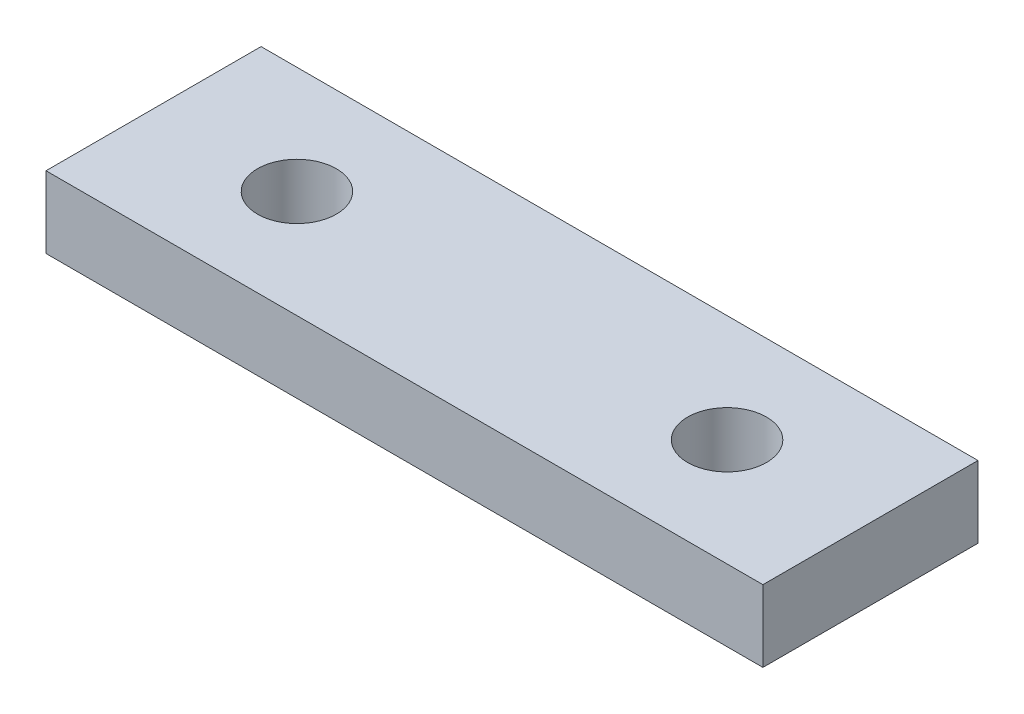
SolidWorks part; units mm, degrees
material "Q235B"
ref_plane "Front Plane" through (0, 0, 0) normal (0, 0, 1) x (1, 0, 0)
ref_plane "Top Plane" through (0, 0, 0) normal (0, 1, 0) x (1, 0, 0)
ref_plane "Right Plane" through (0, 0, 0) normal (1, 0, 0) x (0, 0, -1)
sketch "Sketch1" plane through (0, 0, 0) normal (0, 1, 0) x (1, 0, 0)
  line L1 (50, -15) -> (-50, -15)
  line L2 (50, -15) -> (50, 15)
  line L3 (50, 15) -> (-50, 15)
  line L4 (-50, -15) -> (-50, 15)
  line L5 (50, -15) -> (-50, 15) construction
  line L6 (50, 15) -> (-50, -15) construction
  point P0 (0, 0)
  dimension "D1" = 30
  dimension "D2" = 100
extrude "Boss-Extrude1" add sketch "Sketch1" along normal blind 10
hole_wizard "Ø11.0 (11) Diameter Hole1" positions "Sketch2" profile "Sketch3" hole size "Ø11.0" standard "GB" end condition up to next
sketch "Sketch2" plane through (0, 10, 0) normal (0, 1, 0) x (1, 0, 0)
  line L0 (0, 0) -> (-30, 0) construction
  line L2 (0, 0) -> (0, 15) construction
  line L3 (50, 15) -> (-50, 15) construction
  point P0 (-30, 0)
  point P13 (30, 0)
  dimension "D1" = 60
sketch "Sketch3" plane through (-30, 10, 0) normal (1, 0, 0) x (0, 0, 1)
  line L0 (0, 0) -> (0, 10)
  line L1 (0, 10) -> (5.5, 10)
  line L2 (5.5, 10) -> (5.5, 0)
  line L5 (5.5, 0) -> (0, 0)
  line L11 (0, -6.35) -> (0, 107.95) construction
  dimension "通孔孔直径" = 11
  dimension "通孔孔深度" = 10
